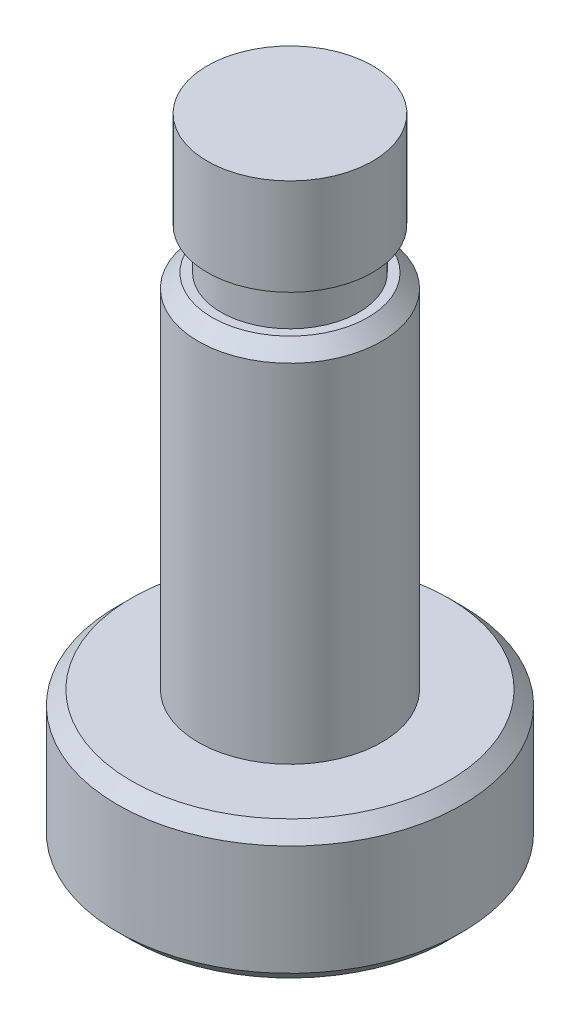
SolidWorks part; units mm, degrees
material "45#"
ref_plane "前视基准面" through (0, 0, 0) normal (0, 0, 1) x (1, 0, 0)
ref_plane "上视基准面" through (0, 0, 0) normal (0, 1, 0) x (1, 0, 0)
ref_plane "右视基准面" through (0, 0, 0) normal (1, 0, 0) x (0, 0, -1)
sketch "草图1" plane through (0, 0, 0) normal (0, 0, 1) x (1, 0, 0)
  line L0 (343.0871, 40.082) -> (343.0871, 78.082) construction
  line L1 (325.5871, 40.082) -> (360.5871, 40.082) construction
  line L2 (349.0871, 78.082) -> (337.0871, 78.082) construction
  line L3 (349.0871, 76.282) -> (349.0871, 69.282)
  line L4 (349.0871, 69.282) -> (348.0871, 69.282)
  line L5 (348.0871, 69.282) -> (348.0871, 66.282)
  line L6 (348.0871, 66.282) -> (349.7371, 66.282)
  line L7 (349.7371, 55.282) -> (349.7371, 67.282) construction
  line L8 (349.7371, 66.282) -> (349.7371, 40.082)
  line L9 (349.7371, 40.082) -> (355.5871, 40.082)
  line L10 (355.5871, 40.082) -> (355.5871, 30.082)
  line L11 (355.5871, 30.082) -> (343.0871, 30.082)
  line L12 (343.0871, 40.082) -> (343.0871, 30.082) construction
  line L13 (292.9371, 67.282) -> (372.9371, 67.282) construction
  line L14 (349.0871, 76.282) -> (343.0871, 76.282)
  line L15 (343.0871, 30.082) -> (343.0871, 76.282)
  dimension "D1" = 10
  dimension "D2" = 25
  dimension "D3" = 12
  dimension "D4" = 1
  dimension "D5" = 3
  dimension "D6" = 1
  dimension "D7" = 7
revolve "旋转1" add sketch "草图1" angle 360 about L15
cosmetic thread "装饰螺纹线1" parameters "D2"=10.106
chamfer "倒角1" distance 1 angle 45 3 edges at (343.0871, 30.082, -12.5) (343.0871, 40.082, -12.5) (343.0871, 66.282, -6.65)
